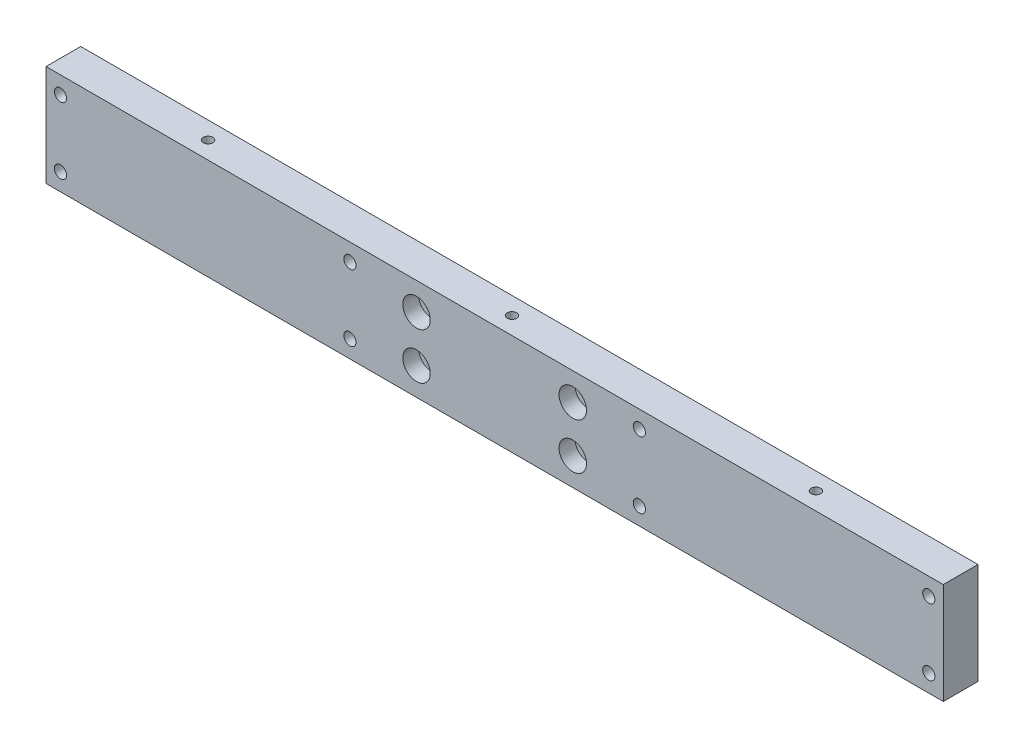
from build123d import *

# Parameters (mm, degrees)
SKETCH_1_W                     = 310
SKETCH_1_H                     = 35
EXTRUDE_1_DEPTH                = 6
HOLE_WIZARD_M5_1_D             = 4.2
PATTERN_LINEAR_2_COUNT         = 4
PATTERN_LINEAR_2_PITCH         = 100
HOLE_WIZARD_M5_1_2_D           = 5.5
HOLE_WIZARD_M5_1_2_CBORE_D     = 9.5
HOLE_WIZARD_M5_1_2_CBORE_DEPTH = 5.5
HOLE_WIZARD_M4_1_D             = 3.3
HOLE_WIZARD_M4_1_DEPTH         = 12.4
HOLE_WIZARD_M4_1_TIP           = 0.991420021


with BuildPart() as part:
    # 草图1 → 凸台-拉伸1 (new, symmetric)
    with BuildSketch(Plane.XY):
        Rectangle(SKETCH_1_W, SKETCH_1_H)
    extrude(amount=EXTRUDE_1_DEPTH, both=True)

    # Hole Wizard M5 _1 (through all)
    with Locations(Plane.XY.offset(6)):
        with Locations((150, 11.5), (150, -11.5)):
            hole_wizard_m5_1 = Hole(HOLE_WIZARD_M5_1_D / 2)

    # 阵列(线性)2: Hole Wizard M5 _1 ×4
    with Locations(*[(-i * PATTERN_LINEAR_2_PITCH, 0, 0) for i in range(1, PATTERN_LINEAR_2_COUNT)]):
        add(hole_wizard_m5_1, mode=Mode.SUBTRACT)

    # Hole Wizard M5 _1 2 (through all)
    with Locations(Plane.XY.offset(6)):
        with Locations((-27, 8), (-27, -8), (27, 8), (27, -8)):
            CounterBoreHole(HOLE_WIZARD_M5_1_2_D / 2, HOLE_WIZARD_M5_1_2_CBORE_D / 2, HOLE_WIZARD_M5_1_2_CBORE_DEPTH)

    # M4 螺纹孔1
    with Locations(Plane(origin=(0, 17.5, 0), x_dir=(1, 0, 0), z_dir=(0, 1, 0))):
        with Locations((105, 0), (0, 0), (-105, 0)):
            Hole(HOLE_WIZARD_M4_1_D / 2, depth=HOLE_WIZARD_M4_1_DEPTH)
            with Locations((0, 0, -(HOLE_WIZARD_M4_1_DEPTH + HOLE_WIZARD_M4_1_TIP / 2))):  # 118° drill point
                Cone(0, HOLE_WIZARD_M4_1_D / 2, HOLE_WIZARD_M4_1_TIP, mode=Mode.SUBTRACT)


solid = part.part
